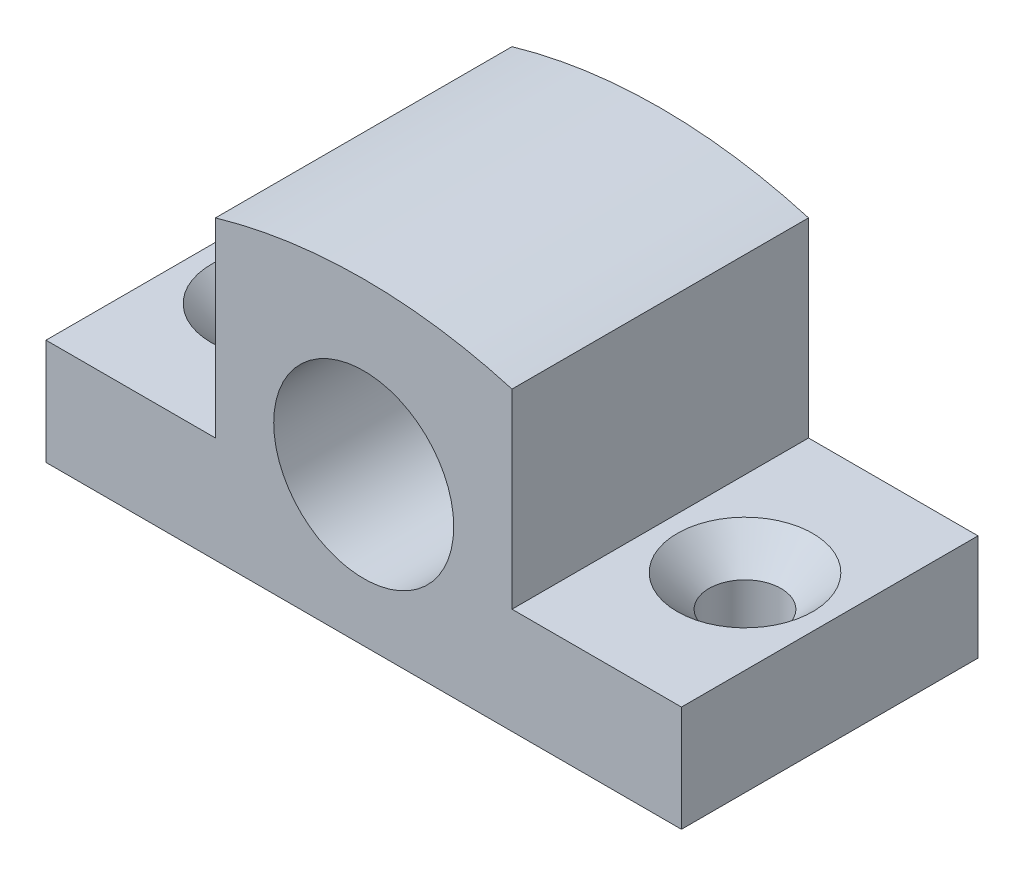
SolidWorks part; units mm, degrees
material "AL6061"
ref_plane "前视基准面" through (0, 0, 0) normal (0, 0, 1) x (1, 0, 0)
ref_plane "上视基准面" through (0, 0, 0) normal (0, 1, 0) x (1, 0, 0)
ref_plane "右视基准面" through (0, 0, 0) normal (1, 0, 0) x (0, 0, -1)
sketch "草图1" plane through (0, 0, 0) normal (0, 0, 1) x (1, 0, 0)
  line L0 (-18.0481, 0) -> (16.7647, 0) construction
  line L1 (0, 9.4652) -> (0, -8.3422) construction
  line L2 (-15, 5) -> (-7, 5)
  line L3 (7, 5) -> (7, 14)
  line L4 (-15, 5) -> (-15, 0)
  line L5 (-15, 0) -> (15, 0)
  line L6 (15, 5) -> (15, 0)
  line L7 (-7, 5) -> (-7, 14)
  line L8 (15, 5) -> (7, 5)
  arc A0 (-7, 14) -> (7, 14) centre (0, -10) cw
  dimension "D4" = 15
  dimension "D5" = 25
  dimension "D1" = 30
  dimension "D2" = 5
  dimension "D3" = 14
extrude "凸台-拉伸1" add sketch "草图1" along normal mid plane 14
hole_wizard "打孔尺寸开槽半沉头螺钉的类型1" positions "草图2" profile "草图3" countersink size "M3" standard "GB" end condition through all
sketch "草图2" plane through (0, 5, 0) normal (0, 1, 0) x (1, 0, 0)
  line L0 (0, 32.3351) -> (0, -35.9769) construction
  line L2 (-16.0611, 0) -> (20.5627, 0) construction
  point P0 (-11, 0)
  point P10 (11, 0)
  dimension "D2" = 22
sketch "草图3" plane through (-11, 5, 0) normal (1, 0, 0) x (0, 0, 1)
  line L0 (0, 0) -> (0, 5)
  line L1 (0, 5) -> (1.7, 5)
  line L2 (1.7, 5) -> (1.7, 1.5)
  line L3 (1.7, 1.5) -> (3.2, 0)
  line L5 (3.2, 0) -> (0, 0)
  line L6 (-1.7, 1.5) -> (-3.2, 0) construction
  line L11 (0, -6.35) -> (0, 107.95) construction
  dimension "通孔孔直径" = 3.4
  dimension "通孔孔深度" = 5
  dimension "近端锥形沉头孔直径" = 6.4
  dimension "近端锥形沉头孔角度" = 90
sketch "草图5" plane through (0, 0, 7) normal (0, 0, 1) x (1, 0, 0)
  line L0 (0, 14.8719) -> (0, -1.5564) construction
  line L1 (-15, 0) -> (15, 0) construction
  circle A0 centre (0, 7) radius 4.25
  dimension "D1" = 7
  dimension "D2" = 8.5
extrude "切除-拉伸1" cut sketch "草图5" against normal through all
